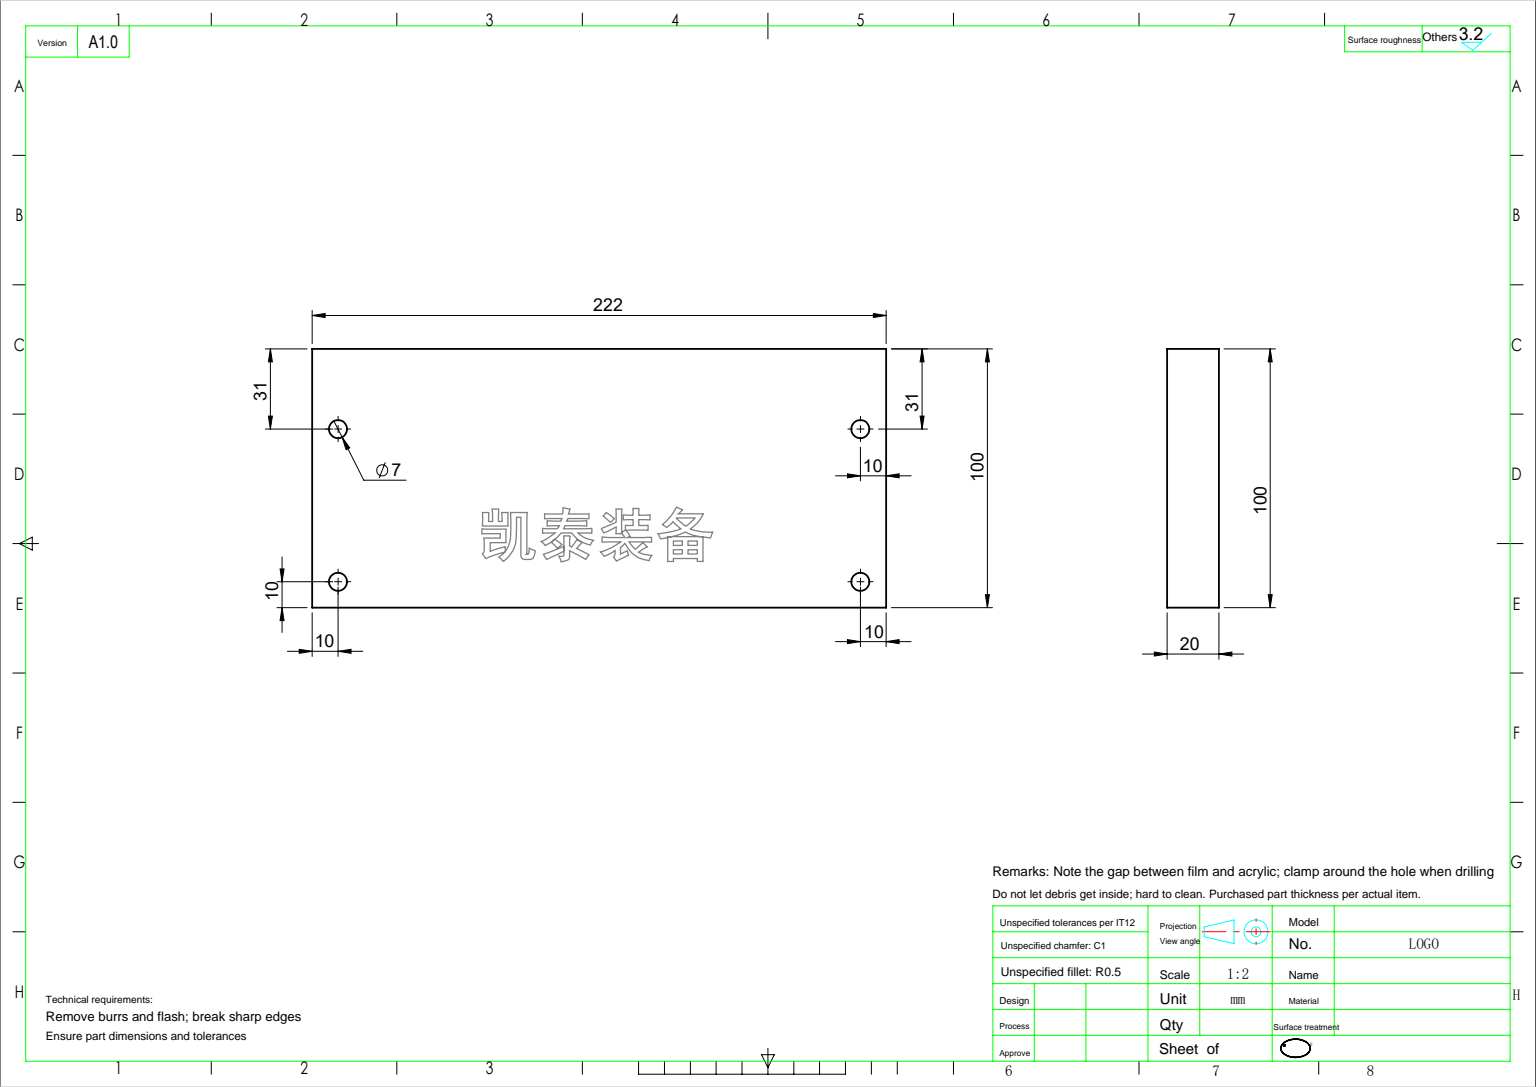
from build123d import *

# Parameters (mm, degrees)
SKETCH_1_W          = 222
SKETCH_1_H          = 100
EXTRUDE_1_DEPTH     = 20
SKETCH_4_R          = 3.5
CUT_EXTRUDE_1_DEPTH = 124.37341691


with BuildPart() as part:
    # 草图1 → 凸台-拉伸1 (new body)
    with BuildSketch(Plane.XY):
        Rectangle(SKETCH_1_W, SKETCH_1_H)
    extrude(amount=EXTRUDE_1_DEPTH)

    # 草图4 → 切除-拉伸1 (cut, through all)
    with BuildSketch(Plane.XY.offset(20)):
        with Locations((-101, 19)):
            Circle(SKETCH_4_R)
        with Locations((-101, -40)):
            Circle(SKETCH_4_R)
        with Locations((101, 19)):
            Circle(SKETCH_4_R)
        with Locations((101, -40)):
            Circle(SKETCH_4_R)
    extrude(amount=-CUT_EXTRUDE_1_DEPTH, mode=Mode.SUBTRACT)


solid = part.part
